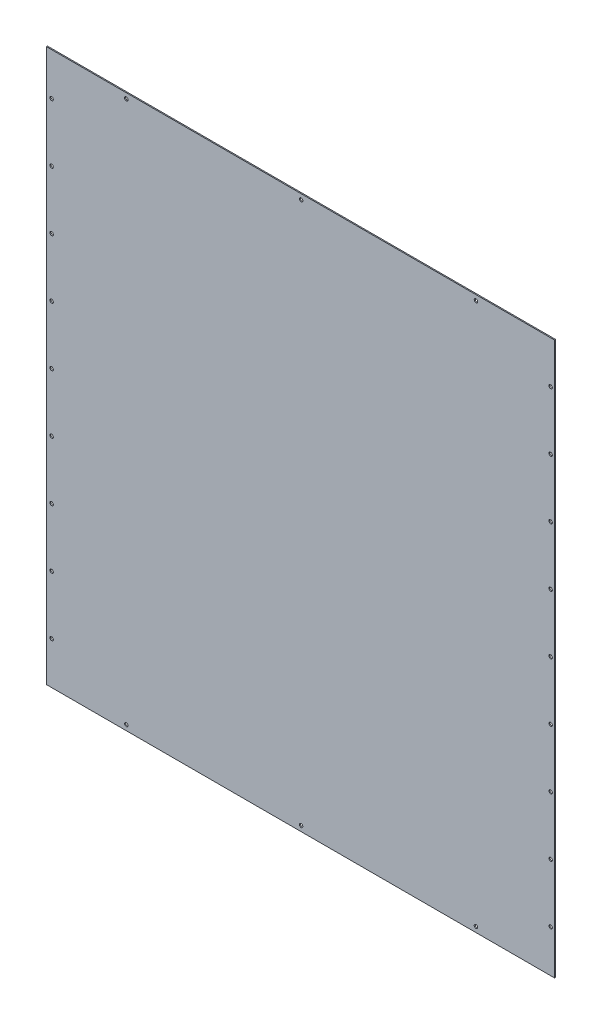
from build123d import *

# Parameters (mm, degrees)
SKETCH_1_W          = 962
SKETCH_1_H          = 1043
SKETCH_1_R          = 3.25
EXTRUDE_1_DEPTH     = 2
SKETCH_2_W          = 2.5
SKETCH_2_H          = 2
CUT_EXTRUDE_1_DEPTH = 1149.570415778


with BuildPart() as part:
    # 草图1 → 凸台-拉伸1 (new body)
    with BuildSketch(Plane.XY):
        Rectangle(SKETCH_1_W, SKETCH_1_H)
        with Locations((-471, 0)):
            Circle(SKETCH_1_R, mode=Mode.SUBTRACT)
        with Locations((-471, -110.375)):
            Circle(SKETCH_1_R, mode=Mode.SUBTRACT)
        with Locations((-471, -220.75)):
            Circle(SKETCH_1_R, mode=Mode.SUBTRACT)
        with Locations((-471, -331.125)):
            Circle(SKETCH_1_R, mode=Mode.SUBTRACT)
        with Locations((-471, -441.5)):
            Circle(SKETCH_1_R, mode=Mode.SUBTRACT)
        with Locations((0, -511.5)):
            Circle(SKETCH_1_R, mode=Mode.SUBTRACT)
        with Locations(Location((0, 511.5, 0), (0, 0, 180))):
            Circle(SKETCH_1_R, mode=Mode.SUBTRACT)
        with Locations(Location((-471, 441.5, 0), (0, 0, 180))):
            Circle(SKETCH_1_R, mode=Mode.SUBTRACT)
        with Locations(Location((-471, 331.125, 0), (0, 0, 180))):
            Circle(SKETCH_1_R, mode=Mode.SUBTRACT)
        with Locations(Location((-471, 220.75, 0), (0, 0, 180))):
            Circle(SKETCH_1_R, mode=Mode.SUBTRACT)
        with Locations(Location((-471, 110.375, 0), (0, 0, 180))):
            Circle(SKETCH_1_R, mode=Mode.SUBTRACT)
        with Locations((471, 110.375)):
            Circle(SKETCH_1_R, mode=Mode.SUBTRACT)
        with Locations((471, 220.75)):
            Circle(SKETCH_1_R, mode=Mode.SUBTRACT)
        with Locations((471, 331.125)):
            Circle(SKETCH_1_R, mode=Mode.SUBTRACT)
        with Locations((471, 441.5)):
            Circle(SKETCH_1_R, mode=Mode.SUBTRACT)
        with Locations(Location((471, -441.5, 0), (0, 0, 180))):
            Circle(SKETCH_1_R, mode=Mode.SUBTRACT)
        with Locations(Location((471, -331.125, 0), (0, 0, 180))):
            Circle(SKETCH_1_R, mode=Mode.SUBTRACT)
        with Locations(Location((471, -220.75, 0), (0, 0, 180))):
            Circle(SKETCH_1_R, mode=Mode.SUBTRACT)
        with Locations(Location((471, -110.375, 0), (0, 0, 180))):
            Circle(SKETCH_1_R, mode=Mode.SUBTRACT)
        with Locations(Location((471, 0, 0), (0, 0, 180))):
            Circle(SKETCH_1_R, mode=Mode.SUBTRACT)
        with Locations((330, -511.5)):
            Circle(SKETCH_1_R, mode=Mode.SUBTRACT)
        with Locations((-330, -511.5)):
            Circle(SKETCH_1_R, mode=Mode.SUBTRACT)
        with Locations(Location((-330, 511.5, 0), (0, 0, 180))):
            Circle(SKETCH_1_R, mode=Mode.SUBTRACT)
        with Locations(Location((330, 511.5, 0), (0, 0, 180))):
            Circle(SKETCH_1_R, mode=Mode.SUBTRACT)
    extrude(amount=EXTRUDE_1_DEPTH)

    # 草图2 → 切除-拉伸1 (cut, through all)
    with BuildSketch(Plane.XZ.offset(521.5)):
        with Locations((479.75, 1)):
            Rectangle(SKETCH_2_W, SKETCH_2_H)
    extrude(amount=-CUT_EXTRUDE_1_DEPTH, mode=Mode.SUBTRACT)


solid = part.part
